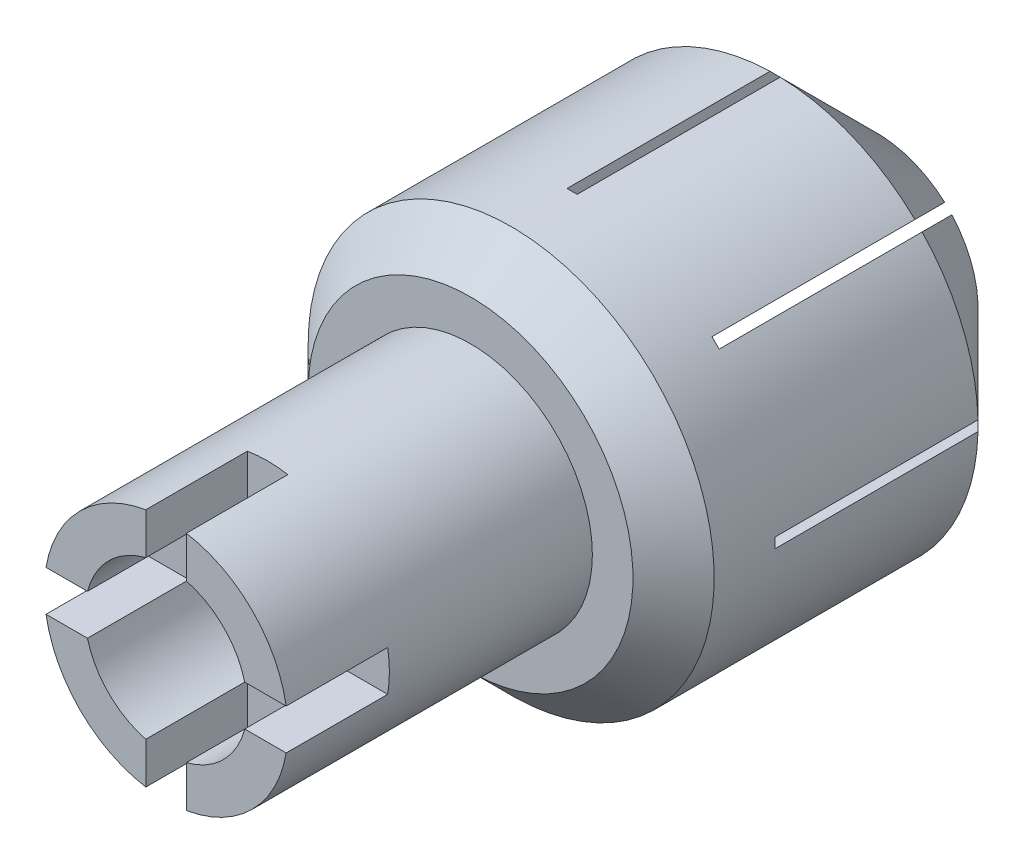
from build123d import *

# Parameters (mm, degrees)
SKETCH1_W          = 2
SKETCH1_H          = 15
CUT_EXTRUDE1_DEPTH = 15
CHAMFER1_SIZE      = 2
CUT_EXTRUDE2_DEPTH = 5


with BuildPart() as part:
    # Sketch1 → Revolve1 (revolve)
    with BuildSketch(Plane(origin=(0, 0, 0), x_dir=(1, 0, 0), z_dir=(0, 1, 0)), mode=Mode.PRIVATE) as revolve1_sk:
        Polygon((3, 20), (3, 0), (4, 0), (6, 0), (10, 0), (10, 15), (5, 20), align=None)
        with Locations((5, -7.5)):
            Rectangle(SKETCH1_W, SKETCH1_H)
    revolve(revolve1_sk.sketch.rotate(Axis((0, 0, -20), (0, 0, 1)), 180), axis=Axis((0, 0, -20), (0, 0, 1)))

    # Sketch2 → Cut-Extrude1 (cut)
    with BuildSketch(Plane(origin=(0, 0, -20), x_dir=(-1, 0, 0), z_dir=(0, 0, -1))):
        with BuildLine():
            ThreePointArc((-9.996874512, 0.25), (-10, 0), (-9.996874512, -0.25))
            Line((-9.996874512, -0.25), (-0.603553391, -0.25))
            Line((-0.603553391, -0.25), (-0.353553391, 0))
            Line((-0.353553391, 0), (-0.603553391, 0.25))
            Line((-0.603553391, 0.25), (-9.996874512, 0.25))
        make_face()
        with BuildLine():
            Line((-0.25, -0.25), (-0.603553391, -0.25))
            Line((-0.603553391, -0.25), (-7.245634453, -6.892081063))
            ThreePointArc((-7.245634453, -6.892081063), (-7.071067812, -7.071067812), (-6.892081063, -7.245634453))
            Line((-6.892081063, -7.245634453), (-0.25, -0.603553391))
            Line((-0.25, -0.603553391), (-0.25, -0.25))
        make_face()
        with BuildLine():
            Line((-7.245634453, 6.892081063), (-0.603553391, 0.25))
            Line((-0.603553391, 0.25), (-0.25, 0.25))
            Line((-0.25, 0.25), (-0.25, 0.603553391))
            Line((-0.25, 0.603553391), (-6.892081063, 7.245634453))
            ThreePointArc((-6.892081063, 7.245634453), (-7.071067812, 7.071067812), (-7.245634453, 6.892081063))
        make_face()
        with BuildLine():
            Line((0, -0.353553391), (-0.25, -0.603553391))
            Line((-0.25, -0.603553391), (-0.25, -9.996874512))
            ThreePointArc((-0.25, -9.996874512), (0, -10), (0.25, -9.996874512))
            Line((0.25, -9.996874512), (0.25, -0.603553391))
            Line((0.25, -0.603553391), (0, -0.353553391))
        make_face()
        with BuildLine():
            Line((-0.25, 9.996874512), (-0.25, 0.603553391))
            Line((-0.25, 0.603553391), (0, 0.353553391))
            Line((0, 0.353553391), (0.25, 0.603553391))
            Line((0.25, 0.603553391), (0.25, 9.996874512))
            ThreePointArc((0.25, 9.996874512), (0, 10), (-0.25, 9.996874512))
        make_face()
        with BuildLine():
            Line((0.603553391, -0.25), (0.25, -0.25))
            Line((0.25, -0.25), (0.25, -0.603553391))
            Line((0.25, -0.603553391), (6.892081063, -7.245634453))
            ThreePointArc((6.892081063, -7.245634453), (7.071067812, -7.071067812), (7.245634453, -6.892081063))
            Line((7.245634453, -6.892081063), (0.603553391, -0.25))
        make_face()
        with BuildLine():
            Line((0.353553391, 0), (0.603553391, -0.25))
            Line((0.603553391, -0.25), (9.996874512, -0.25))
            ThreePointArc((9.996874512, -0.25), (10, 0), (9.996874512, 0.25))
            Line((9.996874512, 0.25), (0.603553391, 0.25))
            Line((0.603553391, 0.25), (0.353553391, 0))
        make_face()
        with BuildLine():
            Line((0.25, 0.603553391), (0.25, 0.25))
            Line((0.25, 0.25), (0.603553391, 0.25))
            Line((0.603553391, 0.25), (7.245634453, 6.892081063))
            ThreePointArc((7.245634453, 6.892081063), (7.071067812, 7.071067812), (6.892081063, 7.245634453))
            Line((6.892081063, 7.245634453), (0.25, 0.603553391))
        make_face()
    extrude(amount=-CUT_EXTRUDE1_DEPTH, mode=Mode.SUBTRACT)

    # Chamfer1
    chamfer1_edges = [part.edges().sort_by_distance(p)[0] for p in [
        (10, 0, 0),
    ]]
    chamfer(chamfer1_edges, length=CHAMFER1_SIZE)

    # Sketch3 → Cut-Extrude2 (cut)
    with BuildSketch(Plane.XY.offset(15)):
        with BuildLine():
            Line((1, 3.872983346), (1, 5.916079783))
            ThreePointArc((1, 5.916079783), (0, 6), (-1, 5.916079783))
            Line((-1, 5.916079783), (-1, 3.872983346))
            ThreePointArc((-1, 3.872983346), (0, 4), (1, 3.872983346))
        make_face()
        with BuildLine():
            ThreePointArc((6, 0), (5.978983137, 0.501757562), (5.916079783, 1))
            Line((5.916079783, 1), (3.872983346, 1))
            ThreePointArc((3.872983346, 1), (3.968118785, 0.50401717), (4, 0))
            ThreePointArc((4, 0), (3.968118785, -0.50401717), (3.872983346, -1))
            Line((3.872983346, -1), (5.916079783, -1))
            ThreePointArc((5.916079783, -1), (5.978983137, -0.501757562), (6, 0))
        make_face()
        with BuildLine():
            ThreePointArc((-1, -5.916079783), (0, -6), (1, -5.916079783))
            Line((1, -5.916079783), (1, -3.872983346))
            ThreePointArc((1, -3.872983346), (0, -4), (-1, -3.872983346))
            Line((-1, -3.872983346), (-1, -5.916079783))
        make_face()
        with BuildLine():
            Line((-3.872983346, 1), (-5.916079783, 1))
            ThreePointArc((-5.916079783, 1), (-6, 0), (-5.916079783, -1))
            Line((-5.916079783, -1), (-3.872983346, -1))
            ThreePointArc((-3.872983346, -1), (-4, 0), (-3.872983346, 1))
        make_face()
    extrude(amount=-CUT_EXTRUDE2_DEPTH, mode=Mode.SUBTRACT)


solid = part.part
